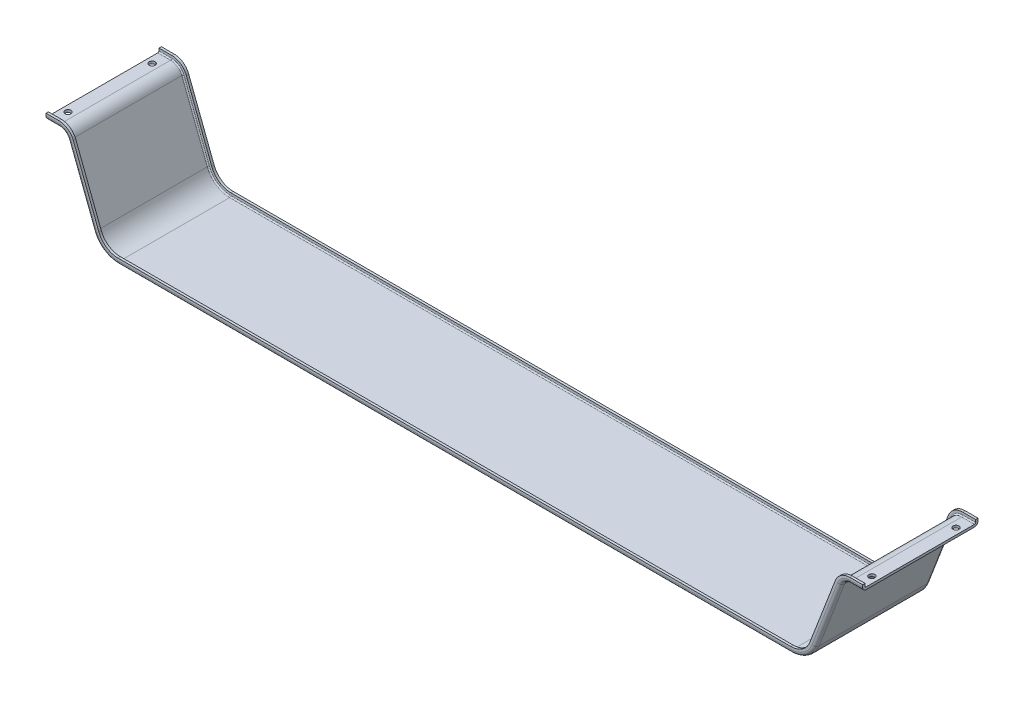
SolidWorks part; units mm, degrees
ref_plane "Front Plane" through (0, 0, 0) normal (0, 0, 1) x (1, 0, 0)
ref_plane "Top Plane" through (0, 0, 0) normal (0, 1, 0) x (1, 0, 0)
ref_plane "Right Plane" through (0, 0, 0) normal (1, 0, 0) x (0, 0, -1)
ref_plane "Plane1" through (0, 107.0541, 0) normal (0, 1, 0) x (1, 0, 0)
sketch "Sketch1" plane through (0, 107.0541, 0) normal (0, 1, 0) x (1, 0, 0)
  line L0 (-1493.1551, 96) -> (-1493.1551, -96)
  line L1 (-1493.1551, -96) -> (-133.8075, -96)
  line L2 (-133.8075, -96) -> (-133.8075, 96)
  line L3 (-133.8075, 96) -> (-1493.1551, 96)
extrude "Boss-Extrude1" add sketch "Sketch1" against normal blind 152.8415
ref_plane "Plane2" through (0, 0, -92) normal (0, 0, -1) x (-1, 0, 0)
sketch "Sketch2" plane through (0, 0, -92) normal (0, 0, -1) x (-1, 0, 0)
  line L0 (168.8075, 107.0541) -> (226, -41.7875)
  line L1 (226, -41.7875) -> (1400.9626, -41.7875)
  line L2 (1400.9626, -41.7875) -> (1458.1551, 107.0541)
  line L3 (1458.1551, 107.0541) -> (168.8075, 107.0541)
extrude "Cut-Extrude1" cut sketch "Sketch2" against normal blind 184
sketch "Sketch3" plane through (0, 107.0541, 0) normal (0, 1, 0) x (-1, 0, 0)
  line L0 (1493.1551, -96) -> (133.8075, -96)
  line L1 (133.8075, -96) -> (133.8075, -92)
  line L2 (133.8075, -92) -> (1493.1551, -92)
  line L3 (1493.1551, -92) -> (1493.1551, -96)
extrude "Boss-Extrude2" add sketch "Sketch3" along normal blind 6
sketch "Sketch4" plane through (0, 107.0541, 0) normal (0, 1, 0) x (-1, 0, 0)
  line L0 (1493.1551, 92) -> (133.8075, 92)
  line L1 (133.8075, 92) -> (133.8075, 96)
  line L2 (133.8075, 96) -> (1493.1551, 96)
  line L3 (1493.1551, 96) -> (1493.1551, 92)
extrude "Boss-Extrude3" add sketch "Sketch4" along normal blind 6
sketch "Sketch5" plane through (0, 0, -96) normal (0, 0, -1) x (-1, 0, 0)
  line L0 (166.0594, 103.0541) -> (133.8075, 103.0541)
  line L1 (133.8075, 103.0541) -> (133.8075, -45.7875)
  line L2 (133.8075, -45.7875) -> (223.2519, -45.7875)
  line L3 (223.2519, -45.7875) -> (166.0594, 103.0541)
extrude "Cut-Extrude2" cut sketch "Sketch5" against normal through all
sketch "Sketch6" plane through (0, 0, -96) normal (0, 0, -1) x (-1, 0, 0)
  line L0 (1454.0329, 113.0541) -> (172.9297, 113.0541)
  line L1 (172.9297, 113.0541) -> (230.1222, -35.7875)
  line L2 (230.1222, -35.7875) -> (1396.8404, -35.7875)
  line L3 (1396.8404, -35.7875) -> (1454.0329, 113.0541)
extrude "Cut-Extrude3" cut sketch "Sketch6" against normal up to next
sketch "Sketch7" plane through (0, 0, 96) normal (0, 0, 1) x (1, 0, 0)
  line L0 (-1460.9032, 103.0541) -> (-1493.1551, 103.0541)
  line L1 (-1493.1551, 103.0541) -> (-1493.1551, -45.7875)
  line L2 (-1493.1551, -45.7875) -> (-1403.7108, -45.7875)
  line L3 (-1403.7108, -45.7875) -> (-1460.9032, 103.0541)
extrude "Cut-Extrude4" cut sketch "Sketch7" against normal through all
sketch "Sketch8" plane through (0, 0, 92) normal (0, 0, -1) x (-1, 0, 0)
  line L0 (1454.0329, 113.0541) -> (172.9297, 113.0541)
  line L1 (172.9297, 113.0541) -> (230.1222, -35.7875)
  line L2 (230.1222, -35.7875) -> (1396.8404, -35.7875)
  line L3 (1396.8404, -35.7875) -> (1454.0329, 113.0541)
extrude "Cut-Extrude5" cut sketch "Sketch8" against normal through all
hole_wizard "Ø10.0 (10) Diameter Hole1" positions "Sketch10" profile "Sketch9" hole size "Ø10.0" standard "ANSI Metric"
sketch "Sketch10" plane through (0, 107.0541, 0) normal (0, 1, 0) x (1, 0, 0)
  point P0 (-144.4372, 70)
  point P1 (-144.4372, -70)
  point P2 (-1482.5254, 70)
  point P3 (-1482.5254, -70)
sketch "Sketch9" plane through (-144.4372, 107.0541, -70) normal (1, 0, 0) x (0, 0, 1)
  line L0 (0, 0) -> (0, 152.8415)
  line L1 (0, 152.8415) -> (5, 152.8415)
  line L2 (5, 152.8415) -> (5, 0)
  line L5 (5, 0) -> (0, 0)
  line L11 (0, -6.35) -> (0, 107.95) construction
  dimension "通孔孔直径" = 10
  dimension "通孔孔深度" = 152.8415
fillet "Fillet1" radius 34 4 edges at (-230.1222, -35.7875, -94) (-1396.8404, -35.7875, 94) (-1396.8404, -35.7875, -94) (-230.1222, -35.7875, 94)
fillet "Fillet2" radius 16 2 edges at (-166.0594, 103.0541, 0) (-1460.9032, 103.0541, 0)
fillet "Fillet3" radius 20 2 edges at (-168.8075, 107.0541, 0) (-1458.1551, 107.0541, 0)
fillet "Fillet4" radius 40 2 edges at (-1400.9626, -41.7875, 0) (-226, -41.7875, 0)
fillet "Fillet5" radius 44 2 edges at (-1403.7108, -45.7875, 0) (-223.2519, -45.7875, 0)
fillet "Fillet6" radius 2 18 edges at (-1482.5254, 107.0541, 92) (-1460.5704, 103.5385, 92) (-144.4372, 107.0541, 92) (-1432.0231, 39.0465, 92) (-166.3922, 103.5385, 92) (-1396.132, -34.7563, 92) (-194.9395, 39.0465, 92) (-813.4813, -41.7875, 92) (-230.8306, -34.7563, 92) (-1482.5254, 107.0541, -92) (-1460.5704, 103.5385, -92) (-144.4372, 107.0541, -92) (-1432.0231, 39.0465, -92) (-166.3922, 103.5385, -92) (-1396.132, -34.7563, -92) (-194.9395, 39.0465, -92) (-813.4813, -41.7875, -92) (-230.8306, -34.7563, -92)
fillet "Fillet7" radius 6 18 edges at (-144.4372, 103.0541, 96) (-1482.5254, 103.0541, 96) (-164.1271, 100.2416, 96) (-1462.8355, 100.2416, 96) (-191.2057, 37.6118, 96) (-1435.757, 37.6118, 96) (-228.5656, -38.0532, 96) (-1398.3971, -38.0532, 96) (-813.4813, -45.7875, 96) (-1482.5254, 103.0541, -96) (-1462.8355, 100.2416, -96) (-1435.757, 37.6118, -96) (-1398.3971, -38.0532, -96) (-813.4813, -45.7875, -96) (-228.5656, -38.0532, -96) (-144.4372, 103.0541, -96) (-191.2057, 37.6118, -96) (-164.1271, 100.2416, -96)
fillet "Fillet8" radius 26 4 edges at (-172.9297, 113.0541, -94) (-1454.0329, 113.0541, 94) (-1454.0329, 113.0541, -94) (-172.9297, 113.0541, 94)
